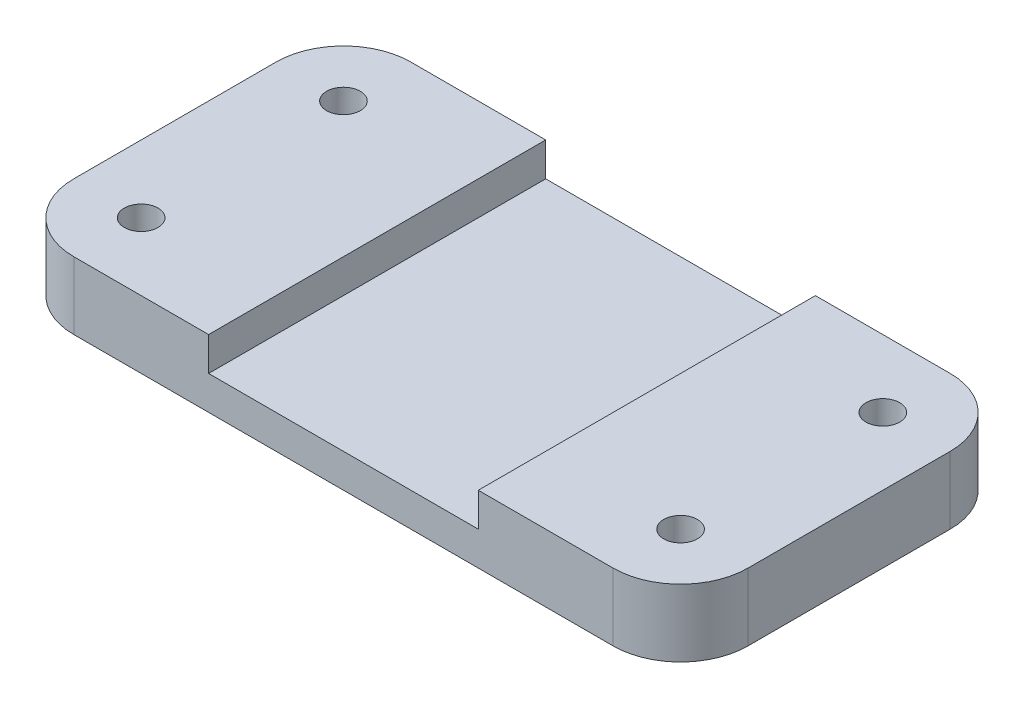
SolidWorks part; units mm, degrees
ref_plane "Front Plane" through (0, 0, 0) normal (0, 0, 1) x (1, 0, 0)
ref_plane "Top Plane" through (0, 0, 0) normal (0, 1, 0) x (1, 0, 0)
ref_plane "Right Plane" through (0, 0, 0) normal (1, 0, 0) x (0, 0, -1)
sketch "Sketch1" plane through (0, 0, 0) normal (0, 1, 0) x (1, 0, 0)
  line L1 (-50, -25) -> (50, -25)
  line L2 (-50, -25) -> (-50, 25)
  line L3 (-50, 25) -> (50, 25)
  line L4 (50, -25) -> (50, 25)
  line L5 (-50, -25) -> (50, 25) construction
  line L6 (-50, 25) -> (50, -25) construction
  point P0 (0, 0)
  dimension "D1" = 100
  dimension "D2" = 50
extrude "Boss-Extrude1" add sketch "Sketch1" along normal blind 10
sketch "Sketch2" plane through (0, 10, 0) normal (0, 1, 0) x (1, 0, 0)
  line L0 (50, 25) -> (-50, 25) construction
  line L1 (-20, -25) -> (20, -25)
  line L2 (-20, -25) -> (-20, 25)
  line L3 (-20, 25) -> (20, 25)
  line L4 (20, -25) -> (20, 25)
  line L5 (-20, -25) -> (20, 25) construction
  line L6 (-20, 25) -> (20, -25) construction
  point P0 (0, 0)
  dimension "D1" = 40
fillet "Fillet1" radius 10 4 edges at (-50, 5, -25) (-50, 5, 25) (50, 5, -25) (50, 5, 25)
hole_wizard "M6 Tapped Hole1" positions "3DSketch1" profile "Sketch3" tap size "M6" standard "GB"
sketch3d "3DSketch1"
  line L0 (-40, 10, 15) -> (-40, 0, 15) construction
  line L1 (-40, 10, -15) -> (-40, 0, -15) construction
  line L2 (40, 10, -15) -> (40, 0, -15) construction
  line L3 (40, 10, 15) -> (40, 0, 15) construction
  point P0 (-40, 10, 15)
  point P4 (-40, 10, -15)
  point P8 (40, 10, -15)
  point P12 (40, 10, 15)
sketch "Sketch3" plane through (-40, 10, 15) normal (1, 0, 0) x (0, 0, 1)
  line L0 (0, 0) -> (0, 15)
  line L1 (0, 15) -> (2.5, 13.4978)
  line L2 (2.5, 13.4978) -> (2.5, 0)
  line L5 (2.5, 0) -> (0, 0)
  line L10 (0, 15) -> (-2.5, 13.4978) construction
  line L11 (0, -6.35) -> (0, 107.95) construction
  dimension "螺纹孔钻头直径" = 5
  dimension "螺纹孔钻头深度" = 15
  dimension "导头角度" = 118
cosmetic thread "Hole Thread1" parameters "D1"=12, "D2"=6
cosmetic thread "Hole Thread2" parameters "D1"=12, "D2"=6
cosmetic thread "Hole Thread3" parameters "D1"=12, "D2"=6
cosmetic thread "Hole Thread4" parameters "D1"=12, "D2"=6
extrude "Cut-Extrude1" cut sketch "Sketch2" against normal blind 5
